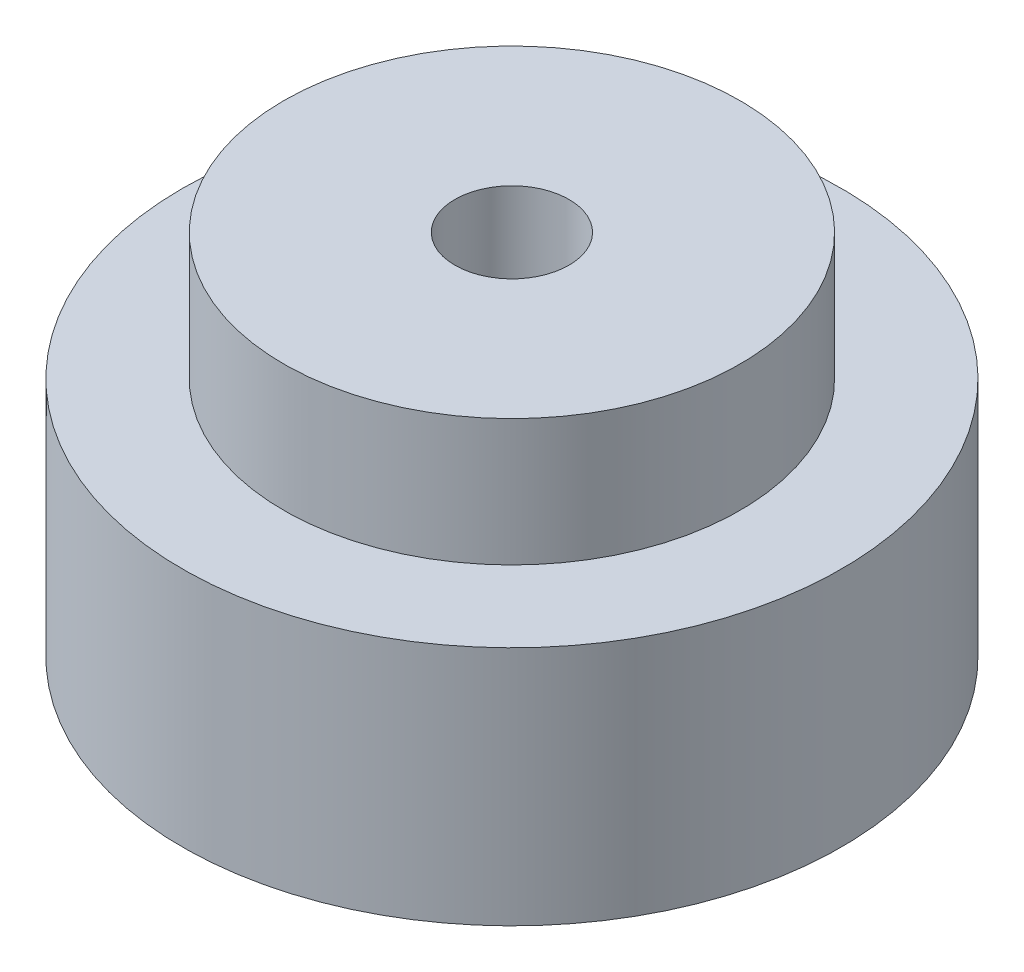
SolidWorks part; units mm, degrees
material "1.0503 (C45)"
ref_plane "Front Plane" through (0, 0, 0) normal (0, 0, 1) x (1, 0, 0)
ref_plane "Top Plane" through (0, 0, 0) normal (0, 1, 0) x (1, 0, 0)
ref_plane "Right Plane" through (0, 0, 0) normal (1, 0, 0) x (0, 0, -1)
sketch "Sketch1" plane through (0, 0, 0) normal (0, 0, 1) x (1, 0, 0)
  line L0 (20, 0) -> (26, 0)
  line L1 (0, 29.7122) -> (0, -13.6211) construction
  line L2 (26, 0) -> (26, 19)
  line L3 (26, 19) -> (18, 19)
  line L4 (18, 19) -> (18, 29)
  line L5 (18, 29) -> (0, 29)
  line L6 (0, 29) -> (0, 17)
  line L7 (-37.6561, 0) -> (41.7766, 0) construction
  line L8 (20, 11) -> (20, 0)
  line L9 (20, 11) -> (5, 17)
  line L10 (5, 17) -> (0, 17)
  dimension "D1" = 52
  dimension "D2" = 36
  dimension "D3" = 19
  dimension "D4" = 29
  dimension "D5" = 10
  dimension "D6" = 40
  dimension "D7" = 11
  dimension "D8" = 12
revolve "Revolve1" add sketch "Sketch1" angle 360 about L1
hole_wizard "M10x1.0 Tapped Hole1" positions "Sketch3" profile "Sketch2" tap size "M10x1.0" standard "GB" end condition up to next
sketch "Sketch3" plane through (0, 29, 0) normal (0, 1, 0) x (1, 0, 0)
  point P0 (0, 0)
sketch "Sketch2" plane through (0, 29, 0) normal (1, 0, 0) x (0, 0, 1)
  line L0 (0, 0) -> (0, 12)
  line L1 (0, 12) -> (4.5, 12)
  line L2 (4.5, 12) -> (4.5, 0)
  line L5 (4.5, 0) -> (0, 0)
  line L11 (0, -6.35) -> (0, 107.95) construction
  dimension "通孔螺纹孔钻头直径" = 9
  dimension "通孔螺纹孔钻头深度" = 12
cosmetic thread "CosmeticThread Hole thread1" parameters "D2"=10
sketch "Sketch4" plane through (0, 0, 0) normal (1, 0, 0) x (0, 0, -1)
  line L0 (0, 41.9025) -> (0, -9.7091) construction
  line L1 (-26, 0) -> (26, 0) construction
  line L2 (-26, 0) -> (26, 0) construction
  circle A0 centre (0, 9) radius 3
  dimension "D2" = 6
  dimension "D1" = 9
extrude "Cut-Extrude1" cut sketch "Sketch4" against normal through all
